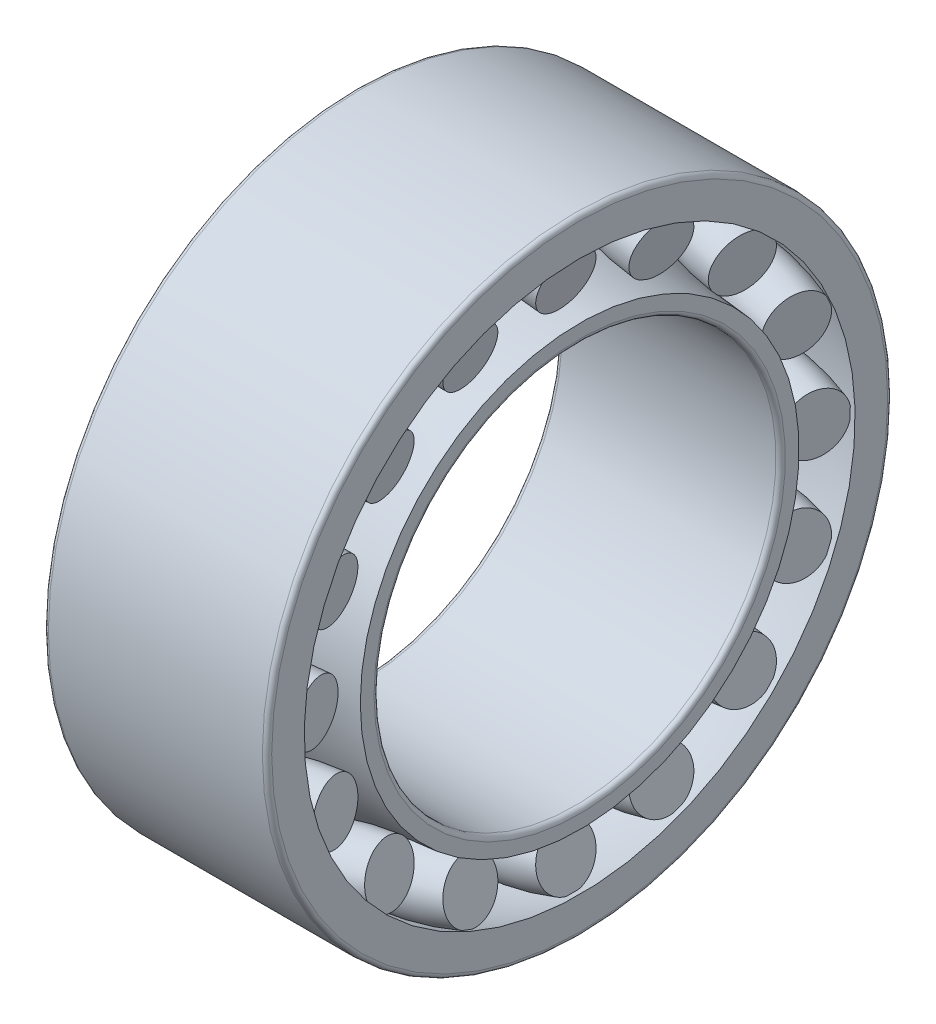
from build123d import *

# Parameters (mm, degrees)
CIRCULAR_PATTERN1_COUNT = 16
FILLET1_R               = 2.1
FILLET2_R               = 2.1


with BuildPart() as part:
    # Sketch1 → Revolve1 (revolve)
    with BuildSketch(Plane.XY, mode=Mode.PRIVATE) as revolve1_sk:
        with BuildLine():
            Line((-8.333333333, 106.666666667), (8.333333333, 106.666666667))
            ThreePointArc((8.333333333, 106.666666667), (28.82803938, 100.779010981), (50, 98.240202425))
            Line((50, 98.240202425), (50, 90))
            Line((50, 90), (-50, 90))
            Line((-50, 90), (-50, 98.240202425))
            ThreePointArc((-50, 98.240202425), (-28.82803938, 100.779010981), (-8.333333333, 106.666666667))
        make_face()
    revolve(revolve1_sk.sketch.rotate(Axis((-50, 0, 0), (1, 0, 0)), 90), axis=Axis((-50, 0, 0), (1, 0, 0)))

    # Fillet2
    fillet2_edges = [part.edges().sort_by_distance(p)[0] for p in [
        (50, 0, -90),
        (-50, 0, -90),
    ]]
    fillet(fillet2_edges, radius=FILLET2_R)


with BuildPart() as body_2:
    # Sketch2 → Revolve2 (revolve)
    with BuildSketch(Plane.XY, mode=Mode.PRIVATE) as revolve2_sk:
        with BuildLine():
            Line((-11.393053417, 119.481327349), (-14.4527735, 132.295988032))
            ThreePointArc((-14.4527735, 132.295988032), (-30.907081139, 129.444441544), (-46.874732157, 124.554689178))
            Line((-46.874732157, 124.554689178), (-43.815012074, 111.740028496))
            Line((-43.815012074, 111.740028496), (-11.393053417, 119.481327349))
        make_face()
    revolve(revolve2_sk.sketch.rotate(Axis((-43.815012074, 111.740028496, 0), (0.9726587597177498, 0.23223896560295143, 0)), 180), axis=Axis((-43.815012074, 111.740028496, 0), (0.9726587597177498, 0.23223896560295143, 0)))


with BuildPart() as body_3:
    # Sketch3 → Revolve3 (revolve)
    with BuildSketch(Plane.XY):
        with BuildLine():
            Line((-50, 123.333333333), (-50, 140))
            Line((-50, 140), (50, 140))
            Line((50, 140), (50, 123.333333333))
            ThreePointArc((50, 123.333333333), (0, 133.083098518), (-50, 123.333333333))
        make_face()
    revolve(axis=Axis((-50, 0, 0), (1, 0, 0)))

    # Fillet1
    fillet1_edges = [body_3.edges().sort_by_distance(p)[0] for p in [
        (-50, -140, 0),
        (50, -140, 0),
    ]]
    fillet(fillet1_edges, radius=FILLET1_R)


with BuildPart() as body_4:
    # Mirror1: mirrored copy
    add(body_2.part.mirror(Plane(origin=(0, 0, 0), x_dir=(0, 0, 1), z_dir=(1, 0, 0))))


with BuildPart() as circular_pattern1_1:
    # Circular-Pattern1: pattern copy
    add(body_4.part.rotate(Axis((0, 0, 0), (1, 0, 0)), 1 * 360 / CIRCULAR_PATTERN1_COUNT))


with BuildPart() as circular_pattern1_2:
    # Circular-Pattern1: pattern copy
    add(body_4.part.rotate(Axis((0, 0, 0), (1, 0, 0)), 2 * 360 / CIRCULAR_PATTERN1_COUNT))


with BuildPart() as circular_pattern1_3:
    # Circular-Pattern1: pattern copy
    add(body_4.part.rotate(Axis((0, 0, 0), (1, 0, 0)), 3 * 360 / CIRCULAR_PATTERN1_COUNT))


with BuildPart() as circular_pattern1_4:
    # Circular-Pattern1: pattern copy
    add(body_4.part.rotate(Axis((0, 0, 0), (1, 0, 0)), 4 * 360 / CIRCULAR_PATTERN1_COUNT))


with BuildPart() as circular_pattern1_5:
    # Circular-Pattern1: pattern copy
    add(body_4.part.rotate(Axis((0, 0, 0), (1, 0, 0)), 5 * 360 / CIRCULAR_PATTERN1_COUNT))


with BuildPart() as circular_pattern1_6:
    # Circular-Pattern1: pattern copy
    add(body_4.part.rotate(Axis((0, 0, 0), (1, 0, 0)), 6 * 360 / CIRCULAR_PATTERN1_COUNT))


with BuildPart() as circular_pattern1_7:
    # Circular-Pattern1: pattern copy
    add(body_4.part.rotate(Axis((0, 0, 0), (1, 0, 0)), 7 * 360 / CIRCULAR_PATTERN1_COUNT))


with BuildPart() as circular_pattern1_8:
    # Circular-Pattern1: pattern copy
    add(body_4.part.rotate(Axis((0, 0, 0), (1, 0, 0)), 8 * 360 / CIRCULAR_PATTERN1_COUNT))


with BuildPart() as circular_pattern1_9:
    # Circular-Pattern1: pattern copy
    add(body_4.part.rotate(Axis((0, 0, 0), (1, 0, 0)), 9 * 360 / CIRCULAR_PATTERN1_COUNT))


with BuildPart() as circular_pattern1_10:
    # Circular-Pattern1: pattern copy
    add(body_4.part.rotate(Axis((0, 0, 0), (1, 0, 0)), 10 * 360 / CIRCULAR_PATTERN1_COUNT))


with BuildPart() as circular_pattern1_11:
    # Circular-Pattern1: pattern copy
    add(body_4.part.rotate(Axis((0, 0, 0), (1, 0, 0)), 11 * 360 / CIRCULAR_PATTERN1_COUNT))


with BuildPart() as circular_pattern1_12:
    # Circular-Pattern1: pattern copy
    add(body_4.part.rotate(Axis((0, 0, 0), (1, 0, 0)), 12 * 360 / CIRCULAR_PATTERN1_COUNT))


with BuildPart() as circular_pattern1_13:
    # Circular-Pattern1: pattern copy
    add(body_4.part.rotate(Axis((0, 0, 0), (1, 0, 0)), 13 * 360 / CIRCULAR_PATTERN1_COUNT))


with BuildPart() as circular_pattern1_14:
    # Circular-Pattern1: pattern copy
    add(body_4.part.rotate(Axis((0, 0, 0), (1, 0, 0)), 14 * 360 / CIRCULAR_PATTERN1_COUNT))


with BuildPart() as circular_pattern1_15:
    # Circular-Pattern1: pattern copy
    add(body_4.part.rotate(Axis((0, 0, 0), (1, 0, 0)), 15 * 360 / CIRCULAR_PATTERN1_COUNT))


with BuildPart() as circular_pattern1_16:
    # Circular-Pattern1: pattern copy
    add(body_2.part.rotate(Axis((0, 0, 0), (1, 0, 0)), 1 * 360 / CIRCULAR_PATTERN1_COUNT))


with BuildPart() as circular_pattern1_17:
    # Circular-Pattern1: pattern copy
    add(body_2.part.rotate(Axis((0, 0, 0), (1, 0, 0)), 2 * 360 / CIRCULAR_PATTERN1_COUNT))


with BuildPart() as circular_pattern1_18:
    # Circular-Pattern1: pattern copy
    add(body_2.part.rotate(Axis((0, 0, 0), (1, 0, 0)), 3 * 360 / CIRCULAR_PATTERN1_COUNT))


with BuildPart() as circular_pattern1_19:
    # Circular-Pattern1: pattern copy
    add(body_2.part.rotate(Axis((0, 0, 0), (1, 0, 0)), 4 * 360 / CIRCULAR_PATTERN1_COUNT))


with BuildPart() as circular_pattern1_20:
    # Circular-Pattern1: pattern copy
    add(body_2.part.rotate(Axis((0, 0, 0), (1, 0, 0)), 5 * 360 / CIRCULAR_PATTERN1_COUNT))


with BuildPart() as circular_pattern1_21:
    # Circular-Pattern1: pattern copy
    add(body_2.part.rotate(Axis((0, 0, 0), (1, 0, 0)), 6 * 360 / CIRCULAR_PATTERN1_COUNT))


with BuildPart() as circular_pattern1_22:
    # Circular-Pattern1: pattern copy
    add(body_2.part.rotate(Axis((0, 0, 0), (1, 0, 0)), 7 * 360 / CIRCULAR_PATTERN1_COUNT))


with BuildPart() as circular_pattern1_23:
    # Circular-Pattern1: pattern copy
    add(body_2.part.rotate(Axis((0, 0, 0), (1, 0, 0)), 8 * 360 / CIRCULAR_PATTERN1_COUNT))


with BuildPart() as circular_pattern1_24:
    # Circular-Pattern1: pattern copy
    add(body_2.part.rotate(Axis((0, 0, 0), (1, 0, 0)), 9 * 360 / CIRCULAR_PATTERN1_COUNT))


with BuildPart() as circular_pattern1_25:
    # Circular-Pattern1: pattern copy
    add(body_2.part.rotate(Axis((0, 0, 0), (1, 0, 0)), 10 * 360 / CIRCULAR_PATTERN1_COUNT))


with BuildPart() as circular_pattern1_26:
    # Circular-Pattern1: pattern copy
    add(body_2.part.rotate(Axis((0, 0, 0), (1, 0, 0)), 11 * 360 / CIRCULAR_PATTERN1_COUNT))


with BuildPart() as circular_pattern1_27:
    # Circular-Pattern1: pattern copy
    add(body_2.part.rotate(Axis((0, 0, 0), (1, 0, 0)), 12 * 360 / CIRCULAR_PATTERN1_COUNT))


with BuildPart() as circular_pattern1_28:
    # Circular-Pattern1: pattern copy
    add(body_2.part.rotate(Axis((0, 0, 0), (1, 0, 0)), 13 * 360 / CIRCULAR_PATTERN1_COUNT))


with BuildPart() as circular_pattern1_29:
    # Circular-Pattern1: pattern copy
    add(body_2.part.rotate(Axis((0, 0, 0), (1, 0, 0)), 14 * 360 / CIRCULAR_PATTERN1_COUNT))


with BuildPart() as circular_pattern1_30:
    # Circular-Pattern1: pattern copy
    add(body_2.part.rotate(Axis((0, 0, 0), (1, 0, 0)), 15 * 360 / CIRCULAR_PATTERN1_COUNT))


solid = Compound([part.part, body_2.part, body_3.part, body_4.part, circular_pattern1_1.part, circular_pattern1_2.part, circular_pattern1_3.part, circular_pattern1_4.part, circular_pattern1_5.part, circular_pattern1_6.part, circular_pattern1_7.part, circular_pattern1_8.part, circular_pattern1_9.part, circular_pattern1_10.part, circular_pattern1_11.part, circular_pattern1_12.part, circular_pattern1_13.part, circular_pattern1_14.part, circular_pattern1_15.part, circular_pattern1_16.part, circular_pattern1_17.part, circular_pattern1_18.part, circular_pattern1_19.part, circular_pattern1_20.part, circular_pattern1_21.part, circular_pattern1_22.part, circular_pattern1_23.part, circular_pattern1_24.part, circular_pattern1_25.part, circular_pattern1_26.part, circular_pattern1_27.part, circular_pattern1_28.part, circular_pattern1_29.part, circular_pattern1_30.part])
